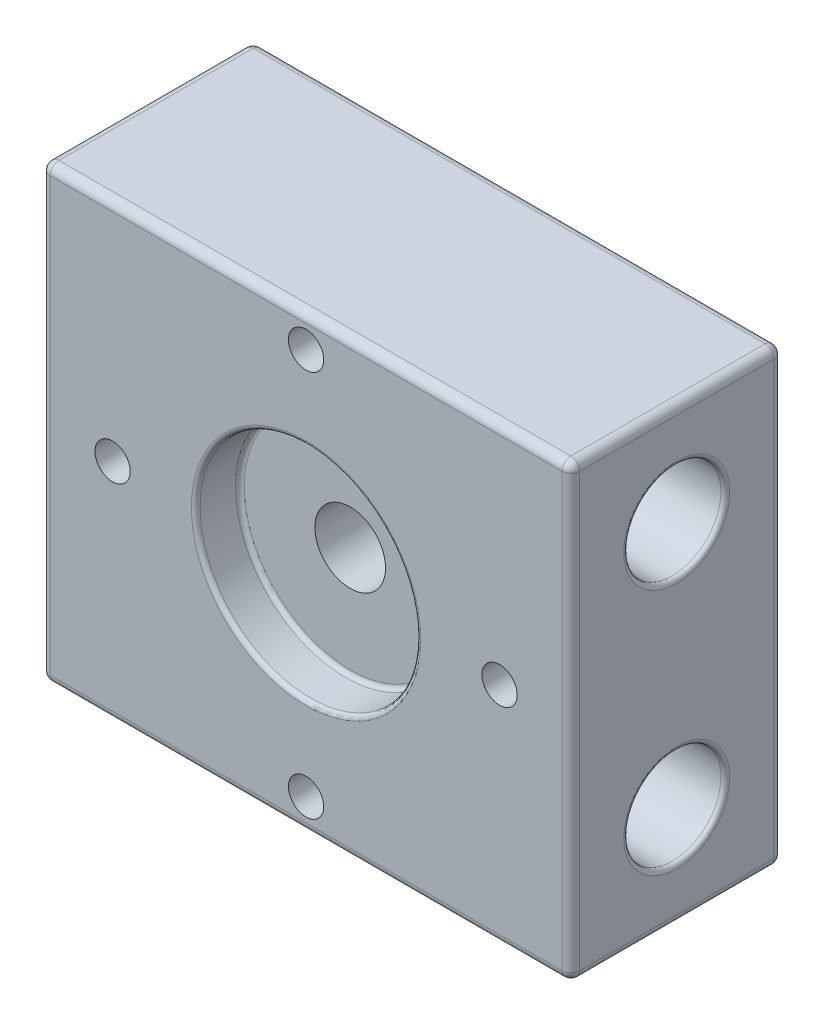
from build123d import *

# Parameters (mm, degrees)
SKETCH1_W           = 60
SKETCH1_H           = 51
BOSS_EXTRUDE1_DEPTH = 12
SKETCH2_R           = 12.5
CUT_EXTRUDE1_DEPTH  = 5
SKETCH3_R           = 5.5
CUT_EXTRUDE2_DEPTH  = 67.289139382
FILLET1_R           = 1
FILLET2_R           = 0.5
SKETCH4_R           = 4
CUT_EXTRUDE3_DEPTH  = 47.111278447
SKETCH5_R           = 2
CUT_EXTRUDE5_DEPTH  = 47.111278447


with BuildPart() as part:
    # Sketch1 → Boss-Extrude1 (new, symmetric)
    with BuildSketch(Plane.XY):
        Rectangle(SKETCH1_W, SKETCH1_H)
    extrude(amount=BOSS_EXTRUDE1_DEPTH, both=True)

    # Sketch2 → Cut-Extrude1 (cut)
    with BuildSketch(Plane.XY.offset(12)):
        Circle(SKETCH2_R)
    extrude(amount=-CUT_EXTRUDE1_DEPTH, mode=Mode.SUBTRACT)

    # Sketch3 → Cut-Extrude2 (cut, through all)
    with BuildSketch(Plane(origin=(30, 0, 0), x_dir=(0, 0, -1), z_dir=(1, 0, 0))):
        with Locations((0, 14)):
            Circle(SKETCH3_R)
        with Locations((0, -14)):
            Circle(SKETCH3_R)
    extrude(amount=-CUT_EXTRUDE2_DEPTH, mode=Mode.SUBTRACT)

    # Fillet1
    fillet1_edges = [part.edges().sort_by_distance(p)[0] for p in [
        (30, 0, 12),
        (0, 25.5, 12),
        (-30, 0, 12),
        (0, 25.5, -12),
        (30, 0, -12),
        (0, -25.5, -12),
        (-30, 0, -12),
        (0, -25.5, 12),
        (-30, 25.5, 0),
        (30, 25.5, 0),
        (30, -25.5, 0),
        (-30, -25.5, 0),
    ]]
    fillet(fillet1_edges, radius=FILLET1_R)

    # Fillet2
    fillet2_edges = [part.edges().sort_by_distance(p)[0] for p in [
        (-12.5, 0, 7),
        (-12.5, 0, 12),
        (-30, 14, 5.5),
        (30, 14, 5.5),
        (-30, -14, 5.5),
        (30, -14, 5.5),
    ]]
    fillet(fillet2_edges, radius=FILLET2_R)

    # Sketch4 → Cut-Extrude3 (cut, through all)
    with BuildSketch(Plane(origin=(0, 0, -12), x_dir=(-1, 0, 0), z_dir=(0, 0, -1))):
        Circle(SKETCH4_R)
    extrude(amount=-CUT_EXTRUDE3_DEPTH, mode=Mode.SUBTRACT)

    # Sketch5 → Cut-Extrude5 (cut, through all)
    with BuildSketch(Plane(origin=(0, 0, -12), x_dir=(-1, 0, 0), z_dir=(0, 0, -1))):
        with Locations((0, -21.920310217)):
            Circle(SKETCH5_R)
        with Locations((-21.920310217, 0)):
            Circle(SKETCH5_R)
        with Locations((0, 21.920310217)):
            Circle(SKETCH5_R)
        with Locations((21.920310217, 0)):
            Circle(SKETCH5_R)
    extrude(amount=-CUT_EXTRUDE5_DEPTH, mode=Mode.SUBTRACT)


solid = part.part
